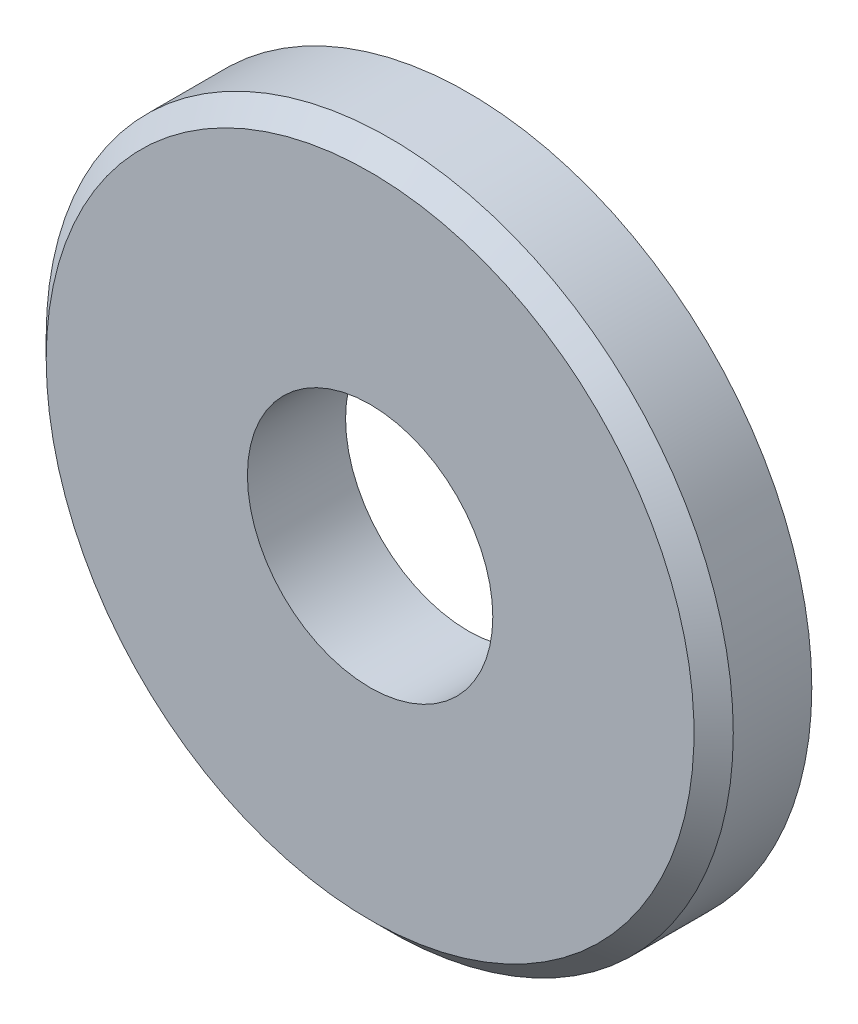
SolidWorks part; units mm, degrees
material "1023 碳钢板 (SS)"
ref_plane "前视基准面" through (0, 0, 0) normal (0, 0, 1) x (1, 0, 0)
ref_plane "上视基准面" through (0, 0, 0) normal (0, 1, 0) x (1, 0, 0)
ref_plane "右视基准面" through (0, 0, 0) normal (1, 0, 0) x (0, 0, -1)
ref_plane "基准面4" through (0, 0, 0) normal (0, -1, 0) x (1, 0, 0)
sketch "草图1" plane through (0, 0, 0) normal (0, -1, 0) x (1, 0, 0)
  line L0 (6.25, 2.5) -> (6.25, -2.5)
  line L1 (6.25, -2.5) -> (17.5, -2.5)
  line L2 (17.5, -2.5) -> (17.5, 1.5)
  line L3 (17.5, 1.5) -> (16.5, 2.5)
  line L4 (16.5, 2.5) -> (6.25, 2.5)
  line L5 (0, 2.5) -> (0, -2.5) construction
revolve "旋转1" add sketch "草图1" angle 360 about L5
